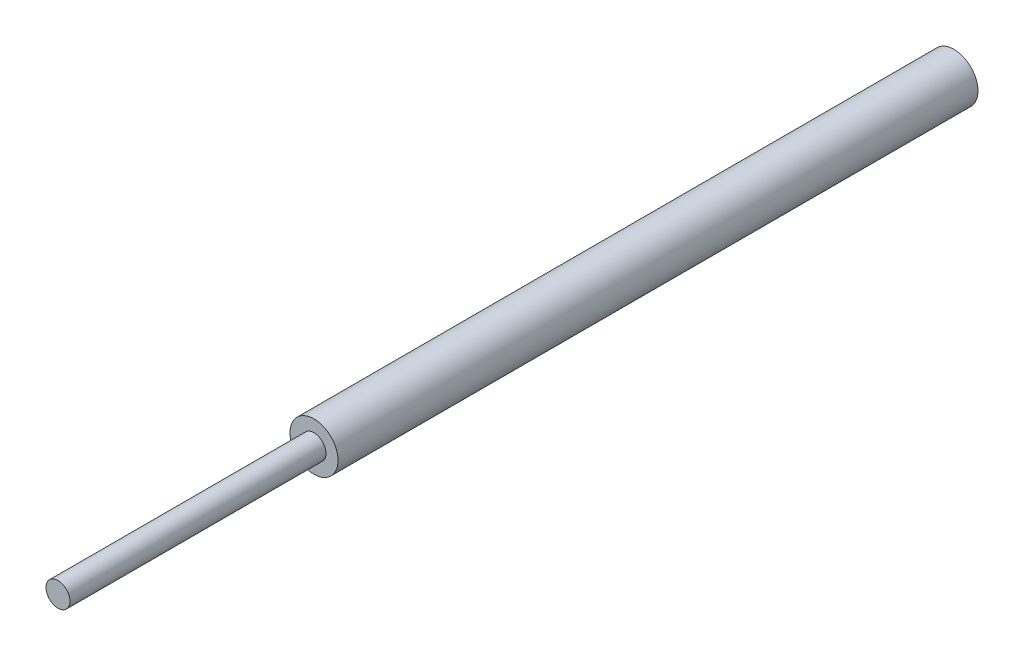
from build123d import *

# Parameters (mm, degrees)
SKETCH1_R           = 1.5
BOSS_EXTRUDE1_DEPTH = 40
SKETCH2_R           = 0.75
BOSS_EXTRUDE2_DEPTH = 16


with BuildPart() as part:
    # Sketch1 → Boss-Extrude1 (new body)
    with BuildSketch(Plane.XY):
        Circle(SKETCH1_R)
    extrude(amount=BOSS_EXTRUDE1_DEPTH)

    # Sketch2 → Boss-Extrude2 (add)
    with BuildSketch(Plane.XY.offset(40)):
        Circle(SKETCH2_R)
    extrude(amount=BOSS_EXTRUDE2_DEPTH)


solid = part.part
